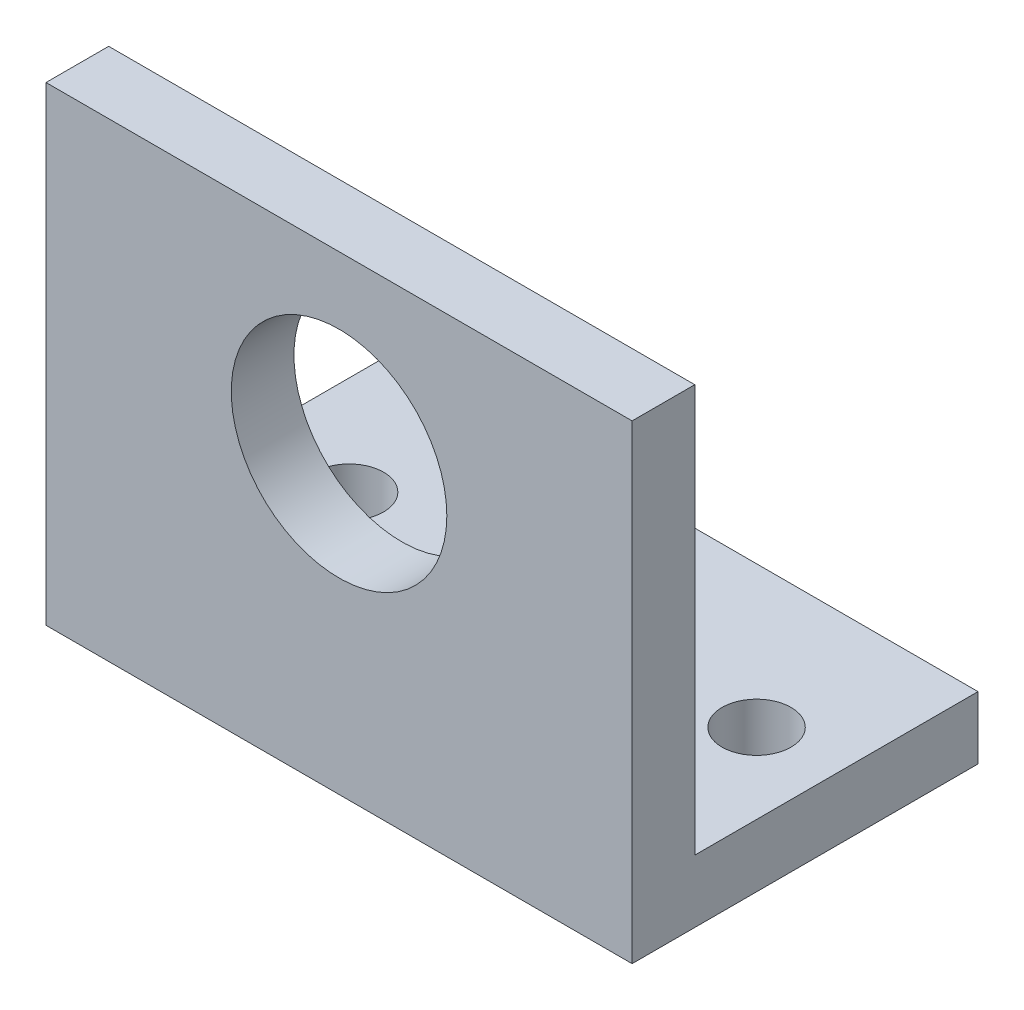
from build123d import *

# Parameters (mm, degrees)
SKETCH1_W           = 18.701399688
SKETCH1_H           = 9.037325038
SKETCH1_R           = 1.1
BOSS_EXTRUDE1_DEPTH = 2
SKETCH2_W           = 18.701399688
SKETCH2_H           = 15
SKETCH2_R           = 3.439163943
BOSS_EXTRUDE2_DEPTH = 2


with BuildPart() as part:
    # Sketch1 → Boss-Extrude1 (new body)
    with BuildSketch(Plane(origin=(0, 0, 0), x_dir=(1, 0, 0), z_dir=(0, 1, 0))):
        Rectangle(SKETCH1_W, SKETCH1_H)
        with Locations(Location((-6.196734059, 0, 0), (0, 0, 270))):
            Circle(SKETCH1_R, mode=Mode.SUBTRACT)
        with Locations(Location((6.803265941, 0, 0), (0, 0, 270))):
            Circle(SKETCH1_R, mode=Mode.SUBTRACT)
    extrude(amount=BOSS_EXTRUDE1_DEPTH)

    # Sketch2 → Boss-Extrude2 (add)
    with BuildSketch(Plane.XY.offset(4.518662519)):
        with Locations((0, 7.5)):
            Rectangle(SKETCH2_W, SKETCH2_H)
        with Locations((0, 9.421314685)):
            Circle(SKETCH2_R, mode=Mode.SUBTRACT)
    extrude(amount=BOSS_EXTRUDE2_DEPTH)


solid = part.part
